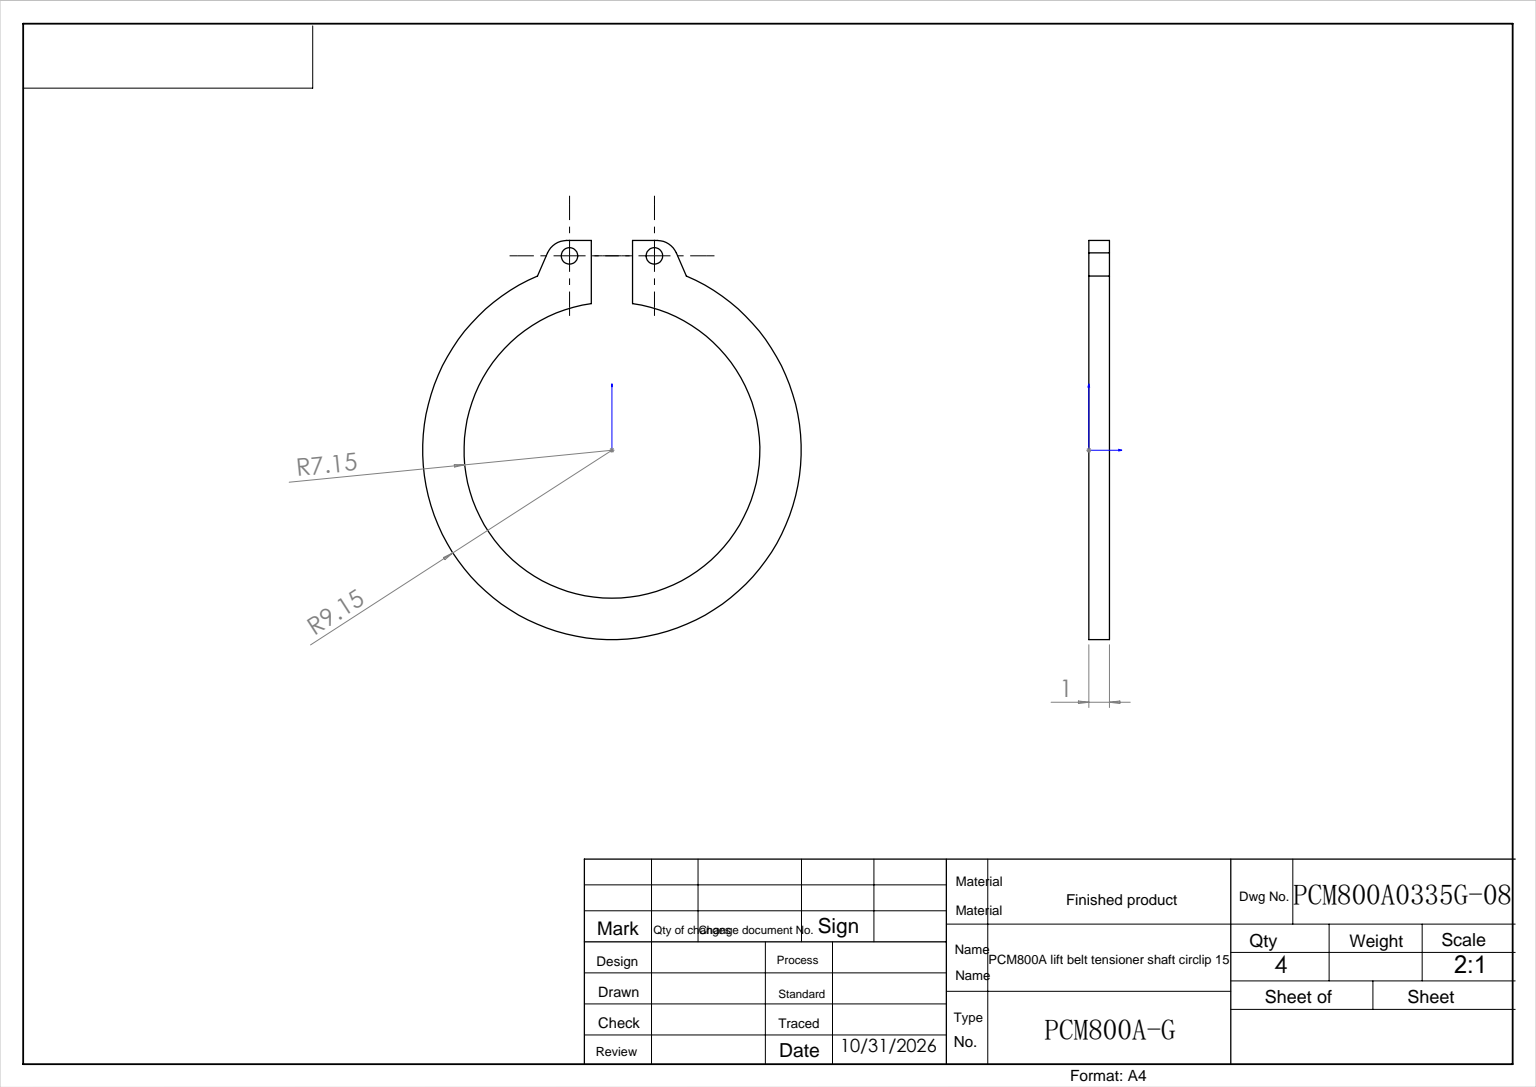
from build123d import *

# Parameters (mm, degrees)
SKETCH_1_R          = 9.15
SKETCH_1_R_2        = 7.15
EXTRUDE_1_DEPTH     = 1
SKETCH_2_W          = 2
SKETCH_2_H          = 11.561648884
CUT_EXTRUDE_1_DEPTH = 13.978636292
EXTRUDE_START       = -1
SKETCH_3_R          = 0.4
EXTRUDE_2_DEPTH     = 1


with BuildPart() as part:
    # 草图1 → 拉伸1 (new body)
    with BuildSketch(Plane(origin=(0, 0, 0), x_dir=(0, 0, -1), z_dir=(1, 0, 0))):
        Circle(SKETCH_1_R)
        Circle(SKETCH_1_R_2, mode=Mode.SUBTRACT)
    extrude(amount=EXTRUDE_1_DEPTH)

    # 草图2 → 切除-拉伸1 (cut, through all)
    with BuildSketch(Plane(origin=(1, 0, 0), x_dir=(0, 0, -1), z_dir=(1, 0, 0))):
        with Locations((0, 5.780824442)):
            Rectangle(SKETCH_2_W, SKETCH_2_H)
    extrude(amount=-CUT_EXTRUDE_1_DEPTH, mode=Mode.SUBTRACT)

    # 草图3 → 拉伸2 (add)
    # profile 1 of 2: a face of its own
    with BuildSketch(Plane(origin=(1, 0, 0), x_dir=(0, 0, -1), z_dir=(1, 0, 0)).offset(EXTRUDE_START)):
        with BuildLine():
            Line((-1, 9.095191037), (-1, 10.12554219))
            Line((-1, 10.12554219), (-2.197020967, 10.125546621))
            ThreePointArc((-2.197020967, 10.125546621), (-2.744657845, 9.962265155), (-3.113455807, 9.525739038))
            Line((-3.113455807, 9.525739038), (-3.599741921, 8.412155378))
            ThreePointArc((-3.599741921, 8.412155378), (-2.325089431, 8.849658702), (-1, 9.095191037))
        make_face()
        with Locations((-2.0521454, 9.383212306)):
            Circle(SKETCH_3_R, mode=Mode.SUBTRACT)
    # profile 2 of 2: a face of its own
    with BuildSketch(Plane(origin=(1, 0, 0), x_dir=(0, 0, -1), z_dir=(1, 0, 0)).offset(EXTRUDE_START)):
        with BuildLine():
            Line((1, 9.095191037), (1, 10.12554219))
            Line((1, 10.12554219), (2.197020967, 10.125546621))
            ThreePointArc((2.197020967, 10.125546621), (2.744657845, 9.962265155), (3.113455807, 9.525739038))
            Line((3.113455807, 9.525739038), (3.599741921, 8.412155378))
            ThreePointArc((3.599741921, 8.412155378), (2.325089431, 8.849658702), (1, 9.095191037))
        make_face()
        with Locations(Location((2.0521454, 9.383212306, 0), (0, 0, 180))):
            Circle(SKETCH_3_R, mode=Mode.SUBTRACT)
    extrude(amount=EXTRUDE_2_DEPTH)


solid = part.part
